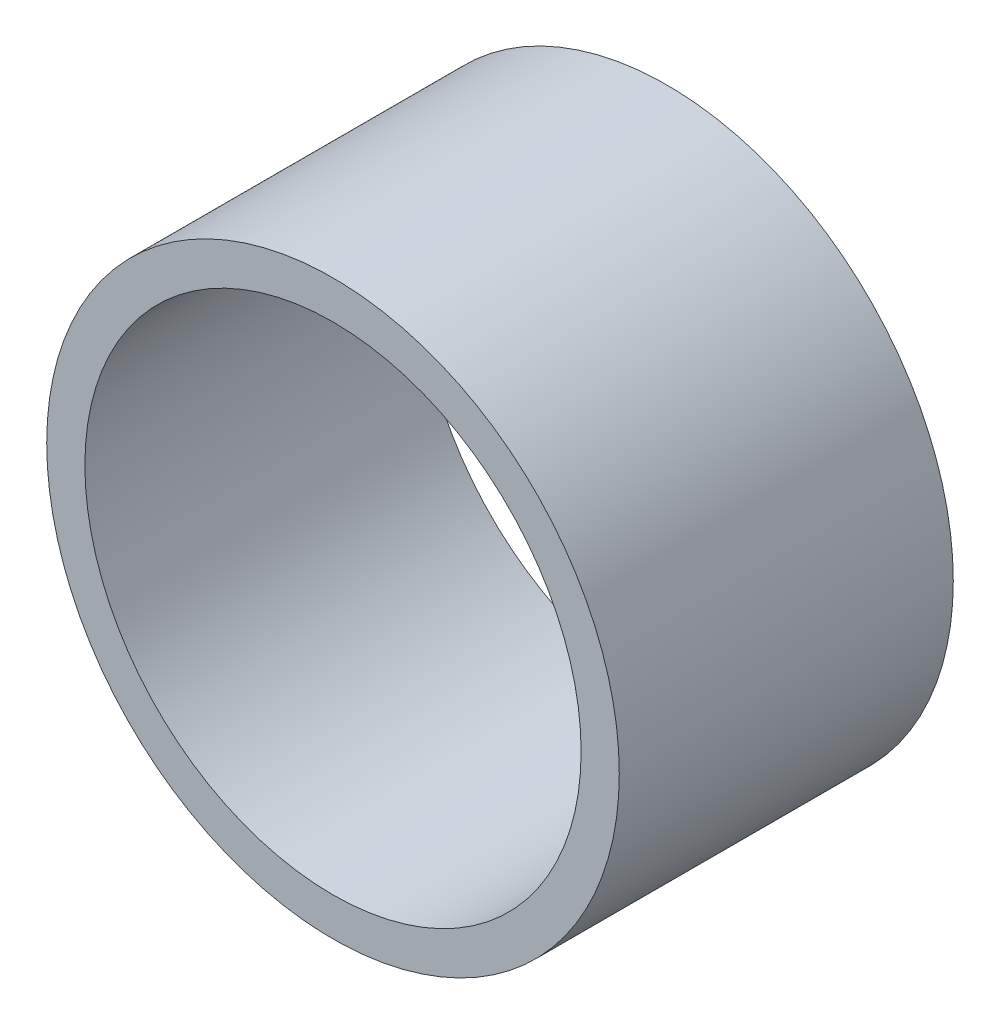
from build123d import *

# Parameters (mm, degrees)
SKETCH1_R           = 15
SKETCH1_R_2         = 13
BOSS_EXTRUDE1_DEPTH = 17.5


with BuildPart() as part:
    # Sketch1 → Boss-Extrude1 (new body)
    with BuildSketch(Plane.XY):
        Circle(SKETCH1_R)
        Circle(SKETCH1_R_2, mode=Mode.SUBTRACT)
    extrude(amount=BOSS_EXTRUDE1_DEPTH)


solid = part.part
